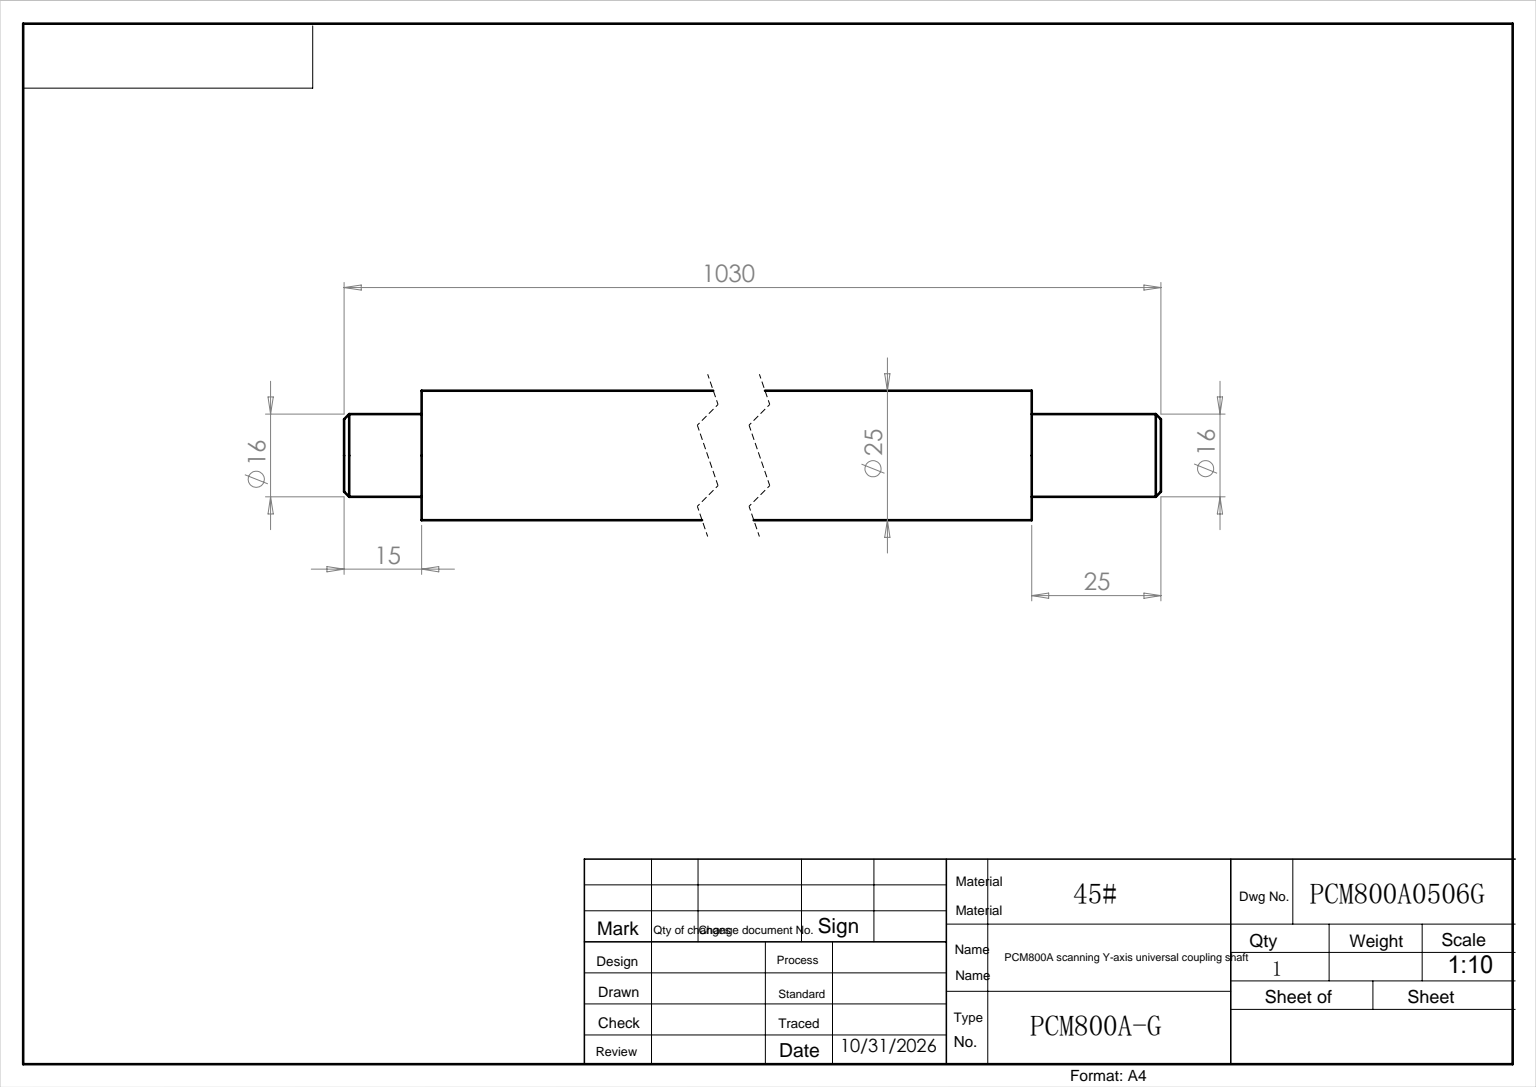
from build123d import *

# Parameters (mm, degrees)
SKETCH_1_R        = 12.5
EXTRUDE_210_DEPTH = 990
SKETCH_2_R        = 8
EXTRUDE_1_DEPTH   = 15
EXTRUDE_START     = 25
SKETCH_3_R        = 8
EXTRUDE_2_DEPTH   = 25
CHAMFER_1_SIZE    = 1


with BuildPart() as part:
    # 草图1 → Extrude 210 (new body)
    with BuildSketch(Plane.XY):
        Circle(SKETCH_1_R)
    extrude(amount=EXTRUDE_210_DEPTH)

    # 草图2 → 凸台-拉伸1 (add)
    with BuildSketch(Plane.XY.offset(990)):
        Circle(SKETCH_2_R)
    extrude(amount=EXTRUDE_1_DEPTH)

    # 草图3 → 凸台-拉伸2 (add)
    with BuildSketch(Plane(origin=(0, 0, 0), x_dir=(-1, 0, 0), z_dir=(0, 0, -1)).offset(EXTRUDE_START)):
        with Locations(Location((0, 0, 0), (0, 0, 180))):
            Circle(SKETCH_3_R)
    extrude(amount=-EXTRUDE_2_DEPTH)

    # 倒角1
    chamfer_1_edges = [part.edges().sort_by_distance(p)[0] for p in [
        (-8, 0, 1005),
        (-8, 0, -25),
    ]]
    chamfer(chamfer_1_edges, length=CHAMFER_1_SIZE)


solid = part.part
